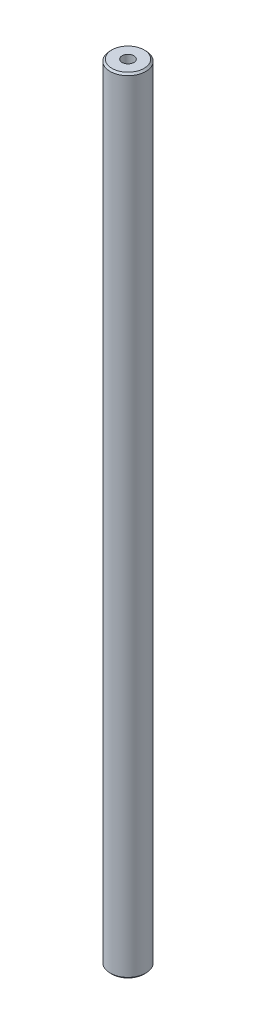
from build123d import *

# Parameters (mm, degrees)
SKETCH1_R             = 5
BOSS_EXTRUDE1_DEPTH   = 110
CHAMFER1_SIZE         = 0.5
M4_TAPPED_HOLE1_D     = 3.3
M4_TAPPED_HOLE1_DEPTH = 10.1
M4_TAPPED_HOLE1_TIP   = 0.991420021
M4_TAPPED_HOLE2_D     = 3.3
M4_TAPPED_HOLE2_DEPTH = 10.1
M4_TAPPED_HOLE2_TIP   = 0.991420021


with BuildPart() as part:
    # Sketch1 → Boss-Extrude1 (new, symmetric)
    with BuildSketch(Plane(origin=(0, 0, 0), x_dir=(1, 0, 0), z_dir=(0, 1, 0))):
        with Locations(Location((0, 0, 0), (0, 0, 270))):
            Circle(SKETCH1_R)
    extrude(amount=BOSS_EXTRUDE1_DEPTH, both=True)

    # Chamfer1
    chamfer1_edges = [part.edges().sort_by_distance(p)[0] for p in [
        (0, -110, -5),
        (0, 110, -5),
    ]]
    chamfer(chamfer1_edges, length=CHAMFER1_SIZE)

    # M4 Tapped Hole1
    with Locations(Plane(origin=(0, 110, 0), x_dir=(1, 0, 0), z_dir=(0, 1, 0))):
        with Locations((0, 0)):
            Hole(M4_TAPPED_HOLE1_D / 2, depth=M4_TAPPED_HOLE1_DEPTH)
            with Locations((0, 0, -(M4_TAPPED_HOLE1_DEPTH + M4_TAPPED_HOLE1_TIP / 2))):  # 118° drill point
                Cone(0, M4_TAPPED_HOLE1_D / 2, M4_TAPPED_HOLE1_TIP, mode=Mode.SUBTRACT)

    # M4 Tapped Hole2
    with Locations(Plane(origin=(0, -110, 0), x_dir=(-1, 0, 0), z_dir=(0, -1, 0))):
        with Locations((0, 0)):
            Hole(M4_TAPPED_HOLE2_D / 2, depth=M4_TAPPED_HOLE2_DEPTH)
            with Locations((0, 0, -(M4_TAPPED_HOLE2_DEPTH + M4_TAPPED_HOLE2_TIP / 2))):  # 118° drill point
                Cone(0, M4_TAPPED_HOLE2_D / 2, M4_TAPPED_HOLE2_TIP, mode=Mode.SUBTRACT)


solid = part.part
